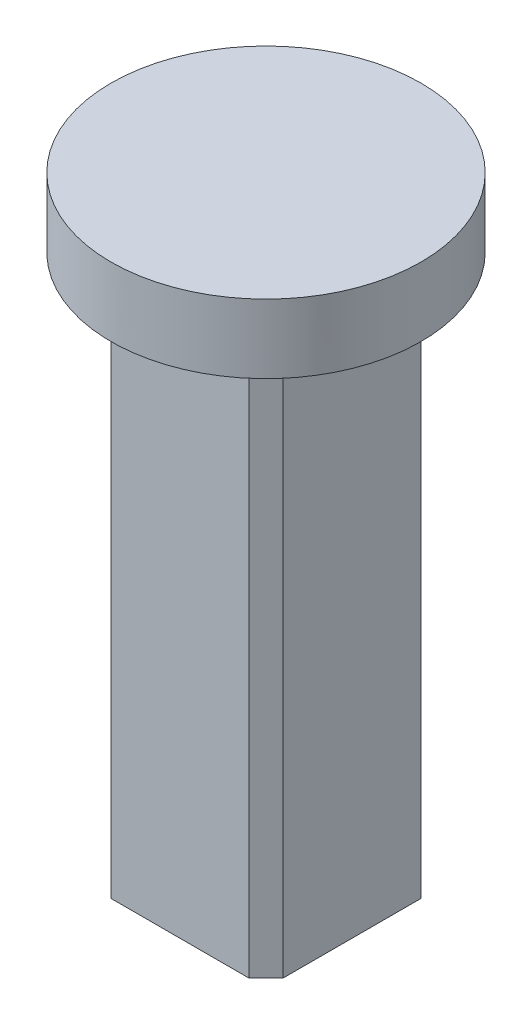
from build123d import *

# Parameters (mm, degrees)
SKETCH_1_R             = 4.5
EXTRUDE_1_DEPTH        = 9
CUT_EXTRUDE_START      = -16
SKETCH_2_R             = 4.5
SKETCH_2_W             = 5
SKETCH_2_H             = 5
CUT_EXTRUDE_1_DEPTH    = 16
HOLE_WIZARD_M3_1_D     = 2.5
HOLE_WIZARD_M3_1_DEPTH = 8.5
HOLE_WIZARD_M3_1_TIP   = 0.751075774
CHAMFER_1_SIZE         = 0.5


with BuildPart() as part:
    # 草图1 → 凸台-拉伸1 (new, symmetric)
    with BuildSketch(Plane(origin=(0, 0, 0), x_dir=(1, 0, 0), z_dir=(0, 1, 0))):
        with Locations(Location((0, 0, 0), (0, 0, 270))):
            Circle(SKETCH_1_R)
    extrude(amount=EXTRUDE_1_DEPTH, both=True)

    # 草图2 → 切除-拉伸1 (cut)
    with BuildSketch(Plane.XZ.offset(9).offset(CUT_EXTRUDE_START)):
        with Locations(Location((0, 0, 0), (0, 0, 270))):
            Circle(SKETCH_2_R)
        Rectangle(SKETCH_2_W, SKETCH_2_H, mode=Mode.SUBTRACT)
    extrude(amount=CUT_EXTRUDE_1_DEPTH, mode=Mode.SUBTRACT)

    # M3 螺纹孔1
    with Locations(Plane(origin=(0, -9, 0), x_dir=(-1, 0, 0), z_dir=(0, -1, 0))):
        with Locations((0, 0)):
            Hole(HOLE_WIZARD_M3_1_D / 2, depth=HOLE_WIZARD_M3_1_DEPTH)
            with Locations((0, 0, -(HOLE_WIZARD_M3_1_DEPTH + HOLE_WIZARD_M3_1_TIP / 2))):  # 118° drill point
                Cone(0, HOLE_WIZARD_M3_1_D / 2, HOLE_WIZARD_M3_1_TIP, mode=Mode.SUBTRACT)

    # 倒角1
    chamfer_1_edges = [part.edges().sort_by_distance(p)[0] for p in [
        (2.5, -1, -2.5),
        (-2.5, -1, -2.5),
        (-2.5, -1, 2.5),
        (2.5, -1, 2.5),
    ]]
    chamfer(chamfer_1_edges, length=CHAMFER_1_SIZE)


solid = part.part
